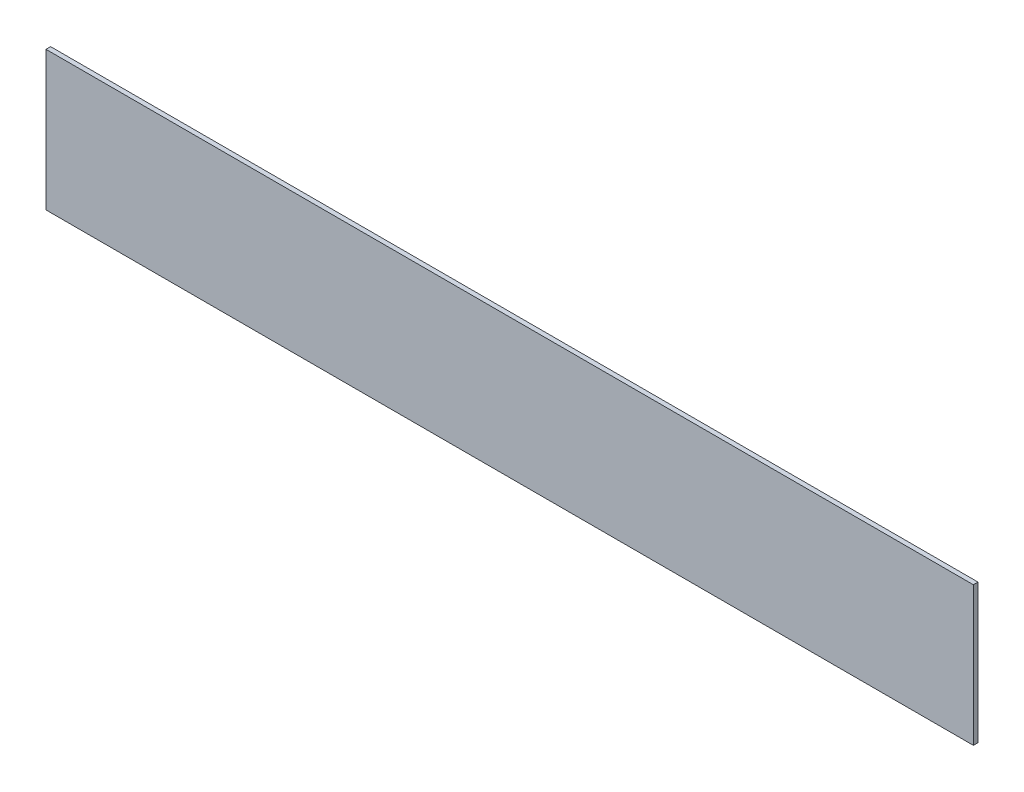
from build123d import *

# Parameters (mm, degrees)
SKETCH1_W           = 1000
SKETCH1_H           = 150
BOSS_EXTRUDE1_DEPTH = 5


with BuildPart() as part:
    # Sketch1 → Boss-Extrude1 (new body)
    with BuildSketch(Plane.XY):
        with Locations((500, 75)):
            Rectangle(SKETCH1_W, SKETCH1_H)
    extrude(amount=BOSS_EXTRUDE1_DEPTH)


solid = part.part
